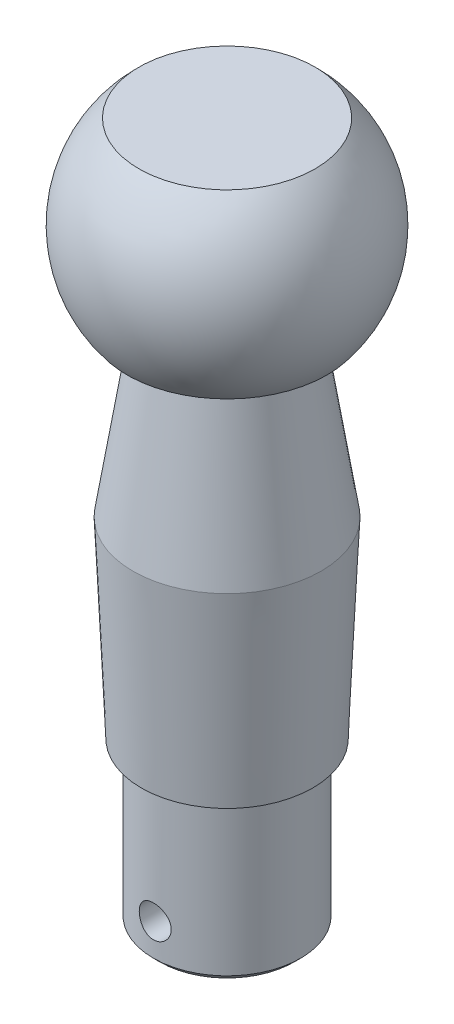
SolidWorks part; units mm, degrees
material "普通碳钢"
ref_plane "前视" through (0, 0, 0) normal (0, 0, 1) x (1, 0, 0)
ref_plane "上视" through (0, 0, 0) normal (0, 1, 0) x (1, 0, 0)
ref_plane "右视" through (0, 0, 0) normal (1, 0, 0) x (0, 0, -1)
sketch "草图1" plane through (0, 0, 0) normal (0, 0, 1) x (1, 0, 0)
  line L0 (-63.0481, 0) -> (65.2329, 0) construction
  line L1 (0, 41.0437) -> (0, -40.2634) construction
  line L2 (0, 14.5) -> (13.775, 14.5)
  line L3 (10.5, -12.5) -> (15.6125, -12.5)
  line L4 (0, 14.5) -> (0, -12.5)
  line L5 (10.5, -12.5) -> (14.7, -39.5)
  line L6 (14.7, -39.5) -> (13.4, -69.5)
  line L7 (13.4, -69.5) -> (11.5, -69.5)
  line L8 (11.5, -69.5) -> (11.5, -94.5)
  line L9 (11.5, -94.5) -> (0, -94.5)
  line L10 (0, -50) -> (0, 50) construction
  line L11 (0, -94.5) -> (0, -12.5)
  arc A0 (15.6125, -12.5) -> (13.775, 14.5) centre (0, 0) ccw
  dimension "D1" = 40
  dimension "D2" = 14.5
  dimension "D3" = 12.5
  dimension "D4" = 10.5
  dimension "D5" = 14.7
  dimension "D6" = 13.4
  dimension "D7" = 11.5
  dimension "D8" = 27
  dimension "D9" = 30
  dimension "D10" = 25
revolve "旋转1" add sketch "草图1" angle 360 about L1
chamfer "倒角1" distance 1 angle 45 1 edges at (0, -94.5, 11.5)
fillet "圆角1" radius 2 1 edges at (0, -12.5, 10.5)
sketch "草图3" plane through (0, 0, 0) normal (0, 0, 1) x (1, 0, 0)
  line L0 (0, -73.8067) -> (0, 73.8067) construction
  line L1 (-10.5, -94.5) -> (10.5, -94.5) construction
  circle A0 centre (0, -88.5) radius 2.5
  dimension "D1" = 6
extrude "切除-拉伸1" cut sketch "草图3" against normal through all both and the other way through all
